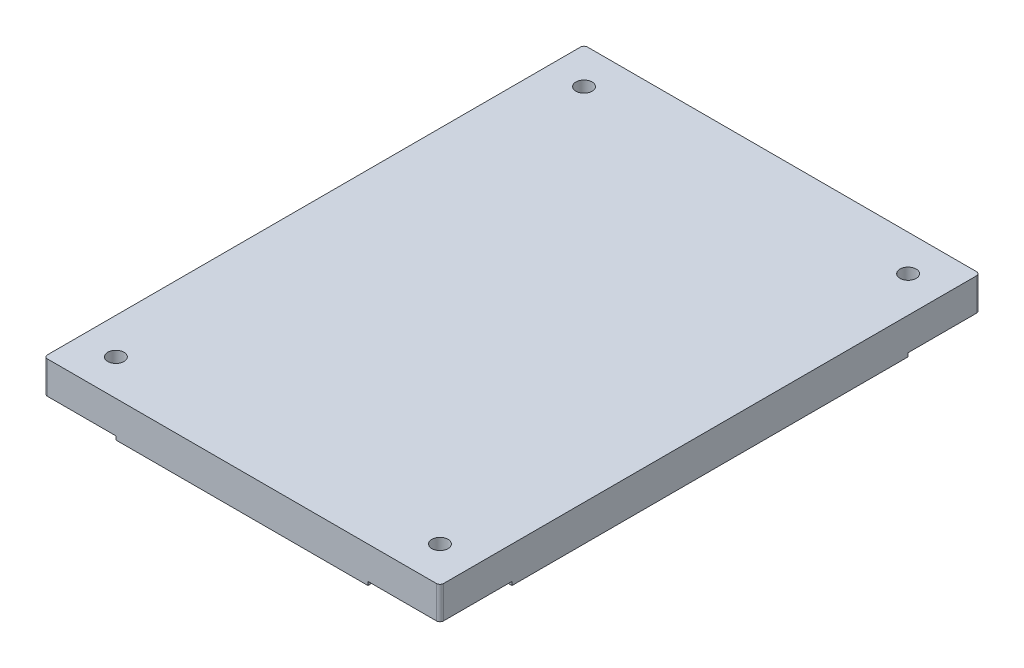
SolidWorks part; units mm, degrees
ref_plane "Front Plane" through (0, 0, 0) normal (0, 0, 1) x (1, 0, 0)
ref_plane "Top Plane" through (0, 0, 0) normal (0, 1, 0) x (1, 0, 0)
ref_plane "Right Plane" through (0, 0, 0) normal (1, 0, 0) x (0, 0, -1)
other "Configuration Table"
sketch "Sketch1" plane through (0, 0, 0) normal (0, 1, 0) x (1, 0, 0)
  line L1 (-55, 75) -> (55, 75)
  line L2 (-55, 75) -> (-55, -75)
  line L3 (-55, -75) -> (55, -75)
  line L4 (55, 75) -> (55, -75)
  line L5 (-55, 75) -> (55, -75) construction
  line L6 (-55, -75) -> (55, 75) construction
  point P0 (0, 0)
  dimension "D1" = 150
  dimension "D2" = 110
extrude "Boss-Extrude1" add sketch "Sketch1" along normal blind 10 contours L2 L3 L4 L1
sketch "Sketch2" plane through (0, 0, 0) normal (0, -1, 0) x (1, 0, 0)
  line L0 (0, 75) -> (0, -75) construction
  line L1 (-55, 75) -> (-35, 75)
  line L2 (-55, 75) -> (-55, 55)
  line L3 (-55, 55) -> (-35, 55)
  line L4 (-35, 75) -> (-35, 55)
  line L5 (-55, 75) -> (55, 75) construction
  line L6 (-55, -75) -> (55, -75) construction
  line L7 (-55, 0) -> (55, 0) construction
  line L8 (-55, -75) -> (-55, 75) construction
  line L9 (55, -75) -> (55, 75) construction
  line L10 (55, 55) -> (35, 55)
  line L11 (35, 75) -> (35, 55)
  line L12 (55, 75) -> (35, 75)
  line L13 (55, 75) -> (55, 55)
  line L14 (55, -75) -> (55, -55)
  line L15 (55, -75) -> (35, -75)
  line L16 (35, -75) -> (35, -55)
  line L17 (55, -55) -> (35, -55)
  line L18 (-55, -55) -> (-35, -55)
  line L19 (-35, -75) -> (-35, -55)
  line L20 (-55, -75) -> (-35, -75)
  line L21 (-55, -75) -> (-55, -55)
  dimension "D1" = 20
  dimension "D2" = 20
extrude "Cut-Extrude1" cut sketch "Sketch2" against normal blind 1
sketch "Sketch3" plane through (0, 1, 0) normal (0, -1, 0) x (1, 0, 0)
  line L0 (-35, 75) -> (-55, 75) construction
  line L1 (-55, 75) -> (-55, 55) construction
  line L2 (55, 75) -> (35, 75) construction
  line L3 (-55, 0) -> (55, 0) construction
  line L4 (-55, -55) -> (-55, 55) construction
  line L5 (55, -55) -> (55, 55) construction
  point P0 (-45, 65)
  point P1 (45, 65)
  point P4 (-45, 75)
  point P7 (-55, 65)
  point P10 (45, 75)
  point P17 (45, -65)
  point P18 (-45, -65)
hole_wizard "Ø4.5 (4.5) Diameter Hole1" positions "Sketch4" profile "Sketch5" hole size "Ø4.5" standard "GB" end condition through all
sketch "Sketch4" plane through (0, 1, 0) normal (0, -1, 0) x (-1, 0, 0)
  point P0 (-45, 65)
  point P3 (45, 65)
  point P6 (45, -65)
  point P9 (-45, -65)
sketch "Sketch5" plane through (45, 1, -65) normal (1, 0, 0) x (0, 0, -1)
  line L0 (0, 0) -> (0, 9)
  line L1 (0, 9) -> (2.25, 9)
  line L2 (2.25, 9) -> (2.25, 0)
  line L5 (2.25, 0) -> (0, 0)
  line L11 (0, -6.35) -> (0, 107.95) construction
  dimension "通孔孔直径" = 4.5
  dimension "通孔孔深度" = 9
fillet "Fillet1" radius 1 4 edges at (35, 0.5, 55) (35, 0.5, -55) (-35, 0.5, 55) (-35, 0.5, -55)
fillet "Fillet2" radius 1 4 edges at (55, 5.5, -75) (55, 5.5, 75) (-55, 5.5, 75) (-55, 5.5, -75)
